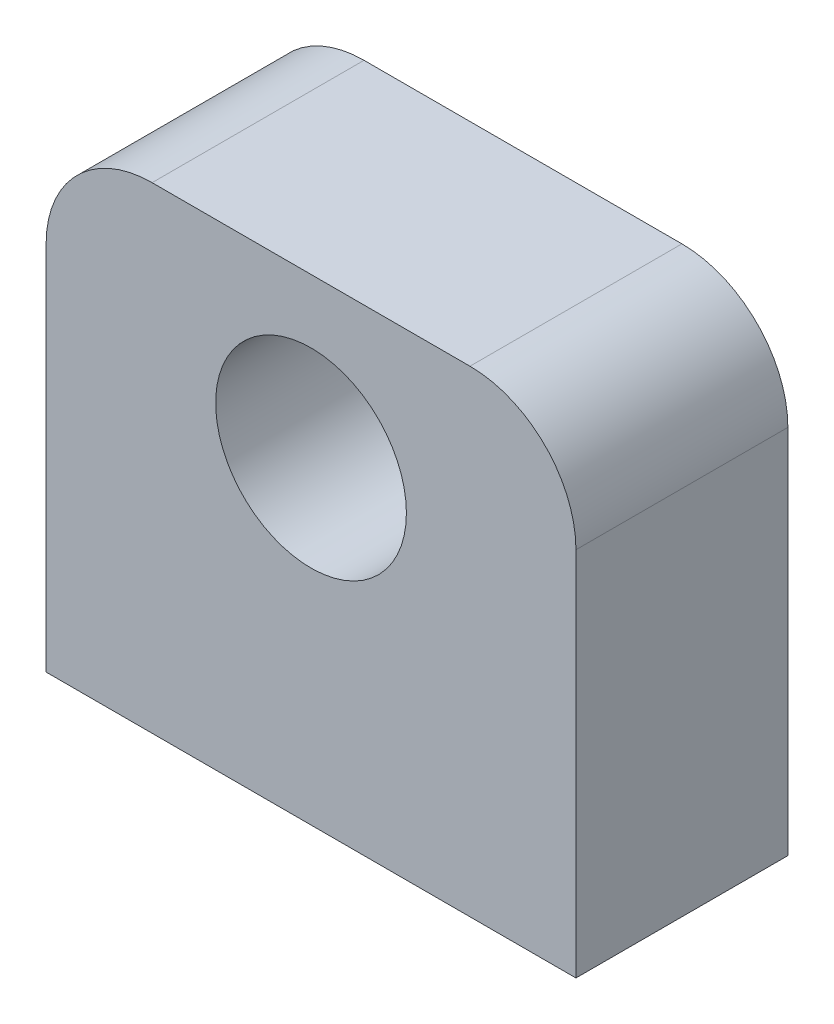
from build123d import *

# Parameters (mm, degrees)
SKETCH1_W           = 50
SKETCH1_H           = 45
SKETCH1_R           = 9
BOSS_EXTRUDE1_DEPTH = 20
FILLET1_R           = 10


with BuildPart() as part:
    # Sketch1 → Boss-Extrude1 (new body)
    with BuildSketch(Plane.XY):
        with Locations((25, 22.5)):
            Rectangle(SKETCH1_W, SKETCH1_H)
        with Locations((25, 30)):
            Circle(SKETCH1_R, mode=Mode.SUBTRACT)
    extrude(amount=BOSS_EXTRUDE1_DEPTH)

    # Fillet1
    fillet1_edges = [part.edges().sort_by_distance(p)[0] for p in [
        (0, 45, 10),
        (50, 45, 10),
    ]]
    fillet(fillet1_edges, radius=FILLET1_R)


solid = part.part
